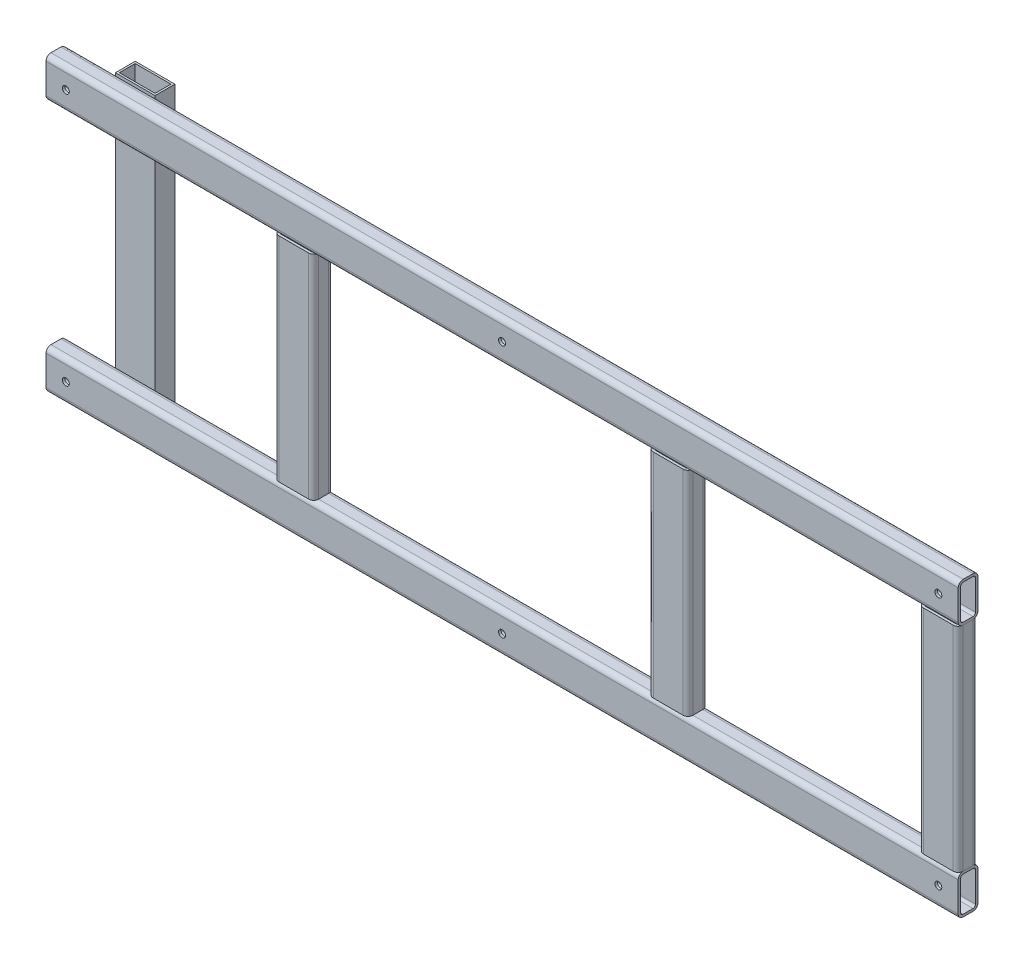
from build123d import *

# Parameters (mm, degrees)
RECT_TUBE_40X20X2_5_1_DEPTH   = 920
RECT_TUBE_40X20X2_5_1_2_DEPTH = 920
RECT_TUBE_40X20X2_5_1_3_DEPTH = 257
RECT_TUBE_40X20X2_5_1_4_DEPTH = 257
RECT_TUBE_40X20X2_5_1_5_DEPTH = 257
M6_CLEARANCE_HOLE1_AT_2_COUNT = 2
M6_CLEARANCE_HOLE1_AT_2_PITCH = 255
M6_CLEARANCE_HOLE1_AT_3_COUNT = 2
M6_CLEARANCE_HOLE1_AT_3_PITCH = 508.551865595
M6_CLEARANCE_HOLE1_AT_4_COUNT = 2
M6_CLEARANCE_HOLE1_AT_4_PITCH = 440
M6_CLEARANCE_HOLE1_AT_5_COUNT = 2
M6_CLEARANCE_HOLE1_AT_5_PITCH = 916.201397074
M6_CLEARANCE_HOLE1_AT_6_COUNT = 2
M6_CLEARANCE_HOLE1_AT_6_PITCH = 880
SKETCH7_W                     = 40
SKETCH7_H                     = 295
BOSS_EXTRUDE1_DEPTH           = 20
SKETCH8_W                     = 36
SKETCH8_H                     = 16
CUT_EXTRUDE1_DEPTH            = 967.604883083


with BuildPart() as part:
    # Sketch1 → Rect Tube 40X20X2.5(1) (new body)
    with BuildSketch(Plane(origin=(0, 0, 0), x_dir=(0, 0, 1), z_dir=(1, 0, 0))):
        with BuildLine():
            Line((-5, -20), (5, -20))
            ThreePointArc((5, -20), (8.535533906, -18.535533906), (10, -15))
            Line((10, -15), (10, 15))
            ThreePointArc((10, 15), (8.535533906, 18.535533906), (5, 20))
            Line((5, 20), (-5, 20))
            ThreePointArc((-5, 20), (-8.535533906, 18.535533906), (-10, 15))
            Line((-10, 15), (-10, -15))
            ThreePointArc((-10, -15), (-8.535533906, -18.535533906), (-5, -20))
        make_face()
        with BuildLine():
            Line((-5, -17.5), (5, -17.5))
            ThreePointArc((5, -17.5), (6.767766953, -16.767766953), (7.5, -15))
            Line((7.5, -15), (7.5, 15))
            ThreePointArc((7.5, 15), (6.767766953, 16.767766953), (5, 17.5))
            Line((5, 17.5), (-5, 17.5))
            ThreePointArc((-5, 17.5), (-6.767766953, 16.767766953), (-7.5, 15))
            Line((-7.5, 15), (-7.5, -15))
            ThreePointArc((-7.5, -15), (-6.767766953, -16.767766953), (-5, -17.5))
        make_face(mode=Mode.SUBTRACT)
    extrude(amount=RECT_TUBE_40X20X2_5_1_DEPTH)


with BuildPart() as body_2:
    # Sketch1 on segment 2 (carried to segment 2) → Rect Tube 40X20X2.5_1 2 (new body)
    with BuildSketch(Plane(origin=(0, -255, 0), x_dir=(0, 0, 1), z_dir=(1, 0, 0))):
        with BuildLine():
            Line((-5, -20), (5, -20))
            ThreePointArc((5, -20), (8.535533906, -18.535533906), (10, -15))
            Line((10, -15), (10, 15))
            ThreePointArc((10, 15), (8.535533906, 18.535533906), (5, 20))
            Line((5, 20), (-5, 20))
            ThreePointArc((-5, 20), (-8.535533906, 18.535533906), (-10, 15))
            Line((-10, 15), (-10, -15))
            ThreePointArc((-10, -15), (-8.535533906, -18.535533906), (-5, -20))
        make_face()
        with BuildLine():
            Line((-5, -17.5), (5, -17.5))
            ThreePointArc((5, -17.5), (6.767766953, -16.767766953), (7.5, -15))
            Line((7.5, -15), (7.5, 15))
            ThreePointArc((7.5, 15), (6.767766953, 16.767766953), (5, 17.5))
            Line((5, 17.5), (-5, 17.5))
            ThreePointArc((-5, 17.5), (-6.767766953, 16.767766953), (-7.5, 15))
            Line((-7.5, 15), (-7.5, -15))
            ThreePointArc((-7.5, -15), (-6.767766953, -16.767766953), (-5, -17.5))
        make_face(mode=Mode.SUBTRACT)
    extrude(amount=RECT_TUBE_40X20X2_5_1_2_DEPTH)

    # Sketch4 → M6 Clearance Hole1 (revolve, cut)
    with BuildSketch(Plane(origin=(20, -255, 10), x_dir=(0, -1, 0), z_dir=(1, 0, 0))):
        Polygon((0, 0), (0, 21.853012167), (3.5, 19.75), (3.5, 0), align=None)
    m6_clearance_hole1 = revolve(axis=Axis((20, -255, 16.35), (0, 0, -1)), mode=Mode.SUBTRACT)

    # M6 Clearance Hole1 at 4: M6 Clearance Hole1 ×2
    with Locations(*[(i * M6_CLEARANCE_HOLE1_AT_4_PITCH, 0, 0) for i in range(1, M6_CLEARANCE_HOLE1_AT_4_COUNT)]):
        add(m6_clearance_hole1, mode=Mode.SUBTRACT)

    # M6 Clearance Hole1 at 6: M6 Clearance Hole1 ×2
    with Locations(*[(i * M6_CLEARANCE_HOLE1_AT_6_PITCH, 0, 0) for i in range(1, M6_CLEARANCE_HOLE1_AT_6_COUNT)]):
        add(m6_clearance_hole1, mode=Mode.SUBTRACT)


with BuildPart() as body_3:
    # Sketch1 on segment 3 (carried to segment 3) → Rect Tube 40X20X2.5_1 3 (new body)
    with BuildSketch(Plane(origin=(900, 1, 0), x_dir=(0, 0, 1), z_dir=(0, -1, 0))):
        with BuildLine():
            Line((-5, -20), (5, -20))
            ThreePointArc((5, -20), (8.535533906, -18.535533906), (10, -15))
            Line((10, -15), (10, 15))
            ThreePointArc((10, 15), (8.535533906, 18.535533906), (5, 20))
            Line((5, 20), (-5, 20))
            ThreePointArc((-5, 20), (-8.535533906, 18.535533906), (-10, 15))
            Line((-10, 15), (-10, -15))
            ThreePointArc((-10, -15), (-8.535533906, -18.535533906), (-5, -20))
        make_face()
        with BuildLine():
            Line((-5, -17.5), (5, -17.5))
            ThreePointArc((5, -17.5), (6.767766953, -16.767766953), (7.5, -15))
            Line((7.5, -15), (7.5, 15))
            ThreePointArc((7.5, 15), (6.767766953, 16.767766953), (5, 17.5))
            Line((5, 17.5), (-5, 17.5))
            ThreePointArc((-5, 17.5), (-6.767766953, 16.767766953), (-7.5, 15))
            Line((-7.5, 15), (-7.5, -15))
            ThreePointArc((-7.5, -15), (-6.767766953, -16.767766953), (-5, -17.5))
        make_face(mode=Mode.SUBTRACT)
    extrude(amount=RECT_TUBE_40X20X2_5_1_3_DEPTH)

    # Rect Tube 40X20X2.5_1 3 end butt 1
    split(bisect_by=Plane(origin=(900, -20, 0), x_dir=(1, 0, 0), z_dir=(0, -1, 0)), keep=Keep.TOP)

    # Rect Tube 40X20X2.5_1 3 end butt 2
    split(bisect_by=Plane(origin=(900, -235, 0), x_dir=(-1, 0, 0), z_dir=(0, 1, 0)), keep=Keep.TOP)


with BuildPart() as body_4:
    # Sketch1 on segment 4 (carried to segment 4) → Rect Tube 40X20X2.5_1 4 (new body)
    with BuildSketch(Plane(origin=(250, 1, 0), x_dir=(0, 0, 1), z_dir=(0, -1, 0))):
        with BuildLine():
            Line((-5, -20), (5, -20))
            ThreePointArc((5, -20), (8.535533906, -18.535533906), (10, -15))
            Line((10, -15), (10, 15))
            ThreePointArc((10, 15), (8.535533906, 18.535533906), (5, 20))
            Line((5, 20), (-5, 20))
            ThreePointArc((-5, 20), (-8.535533906, 18.535533906), (-10, 15))
            Line((-10, 15), (-10, -15))
            ThreePointArc((-10, -15), (-8.535533906, -18.535533906), (-5, -20))
        make_face()
        with BuildLine():
            Line((-5, -17.5), (5, -17.5))
            ThreePointArc((5, -17.5), (6.767766953, -16.767766953), (7.5, -15))
            Line((7.5, -15), (7.5, 15))
            ThreePointArc((7.5, 15), (6.767766953, 16.767766953), (5, 17.5))
            Line((5, 17.5), (-5, 17.5))
            ThreePointArc((-5, 17.5), (-6.767766953, 16.767766953), (-7.5, 15))
            Line((-7.5, 15), (-7.5, -15))
            ThreePointArc((-7.5, -15), (-6.767766953, -16.767766953), (-5, -17.5))
        make_face(mode=Mode.SUBTRACT)
    extrude(amount=RECT_TUBE_40X20X2_5_1_4_DEPTH)

    # Rect Tube 40X20X2.5_1 4 end butt 1
    split(bisect_by=Plane(origin=(250, -20, 0), x_dir=(1, 0, 0), z_dir=(0, -1, 0)), keep=Keep.TOP)

    # Rect Tube 40X20X2.5_1 4 end butt 2
    split(bisect_by=Plane(origin=(250, -235, 0), x_dir=(-1, 0, 0), z_dir=(0, 1, 0)), keep=Keep.TOP)


with BuildPart() as body_5:
    # Sketch1 on segment 5 (carried to segment 5) → Rect Tube 40X20X2.5_1 5 (new body)
    with BuildSketch(Plane(origin=(627.472616431, 1, 0), x_dir=(0, 0, 1), z_dir=(0, -1, 0))):
        with BuildLine():
            Line((-5, -20), (5, -20))
            ThreePointArc((5, -20), (8.535533906, -18.535533906), (10, -15))
            Line((10, -15), (10, 15))
            ThreePointArc((10, 15), (8.535533906, 18.535533906), (5, 20))
            Line((5, 20), (-5, 20))
            ThreePointArc((-5, 20), (-8.535533906, 18.535533906), (-10, 15))
            Line((-10, 15), (-10, -15))
            ThreePointArc((-10, -15), (-8.535533906, -18.535533906), (-5, -20))
        make_face()
        with BuildLine():
            Line((-5, -17.5), (5, -17.5))
            ThreePointArc((5, -17.5), (6.767766953, -16.767766953), (7.5, -15))
            Line((7.5, -15), (7.5, 15))
            ThreePointArc((7.5, 15), (6.767766953, 16.767766953), (5, 17.5))
            Line((5, 17.5), (-5, 17.5))
            ThreePointArc((-5, 17.5), (-6.767766953, 16.767766953), (-7.5, 15))
            Line((-7.5, 15), (-7.5, -15))
            ThreePointArc((-7.5, -15), (-6.767766953, -16.767766953), (-5, -17.5))
        make_face(mode=Mode.SUBTRACT)
    extrude(amount=RECT_TUBE_40X20X2_5_1_5_DEPTH)

    # Rect Tube 40X20X2.5_1 5 end butt 1
    split(bisect_by=Plane(origin=(627.472616431, -20, 0), x_dir=(1, 0, 0), z_dir=(0, -1, 0)), keep=Keep.TOP)

    # Rect Tube 40X20X2.5_1 5 end butt 2
    split(bisect_by=Plane(origin=(627.472616431, -235, 0), x_dir=(-1, 0, 0), z_dir=(0, 1, 0)), keep=Keep.TOP)


with BuildPart() as part_1:
    add(part.part)

    # M6 Clearance Hole1 at 2: M6 Clearance Hole1 ×2
    with Locations(*[(0, i * M6_CLEARANCE_HOLE1_AT_2_PITCH, 0) for i in range(1, M6_CLEARANCE_HOLE1_AT_2_COUNT)]):
        add(m6_clearance_hole1, mode=Mode.SUBTRACT)

    # M6 Clearance Hole1 at 3: M6 Clearance Hole1 ×2
    with Locations(*[Vector(0.8652018206350236, 0.5014237824134796, 0) * (i * M6_CLEARANCE_HOLE1_AT_3_PITCH) for i in range(1, M6_CLEARANCE_HOLE1_AT_3_COUNT)]):
        add(m6_clearance_hole1, mode=Mode.SUBTRACT)

    # M6 Clearance Hole1 at 5: M6 Clearance Hole1 ×2
    with Locations(*[Vector(0.9604875116001456, 0.2783230857477695, 0) * (i * M6_CLEARANCE_HOLE1_AT_5_PITCH) for i in range(1, M6_CLEARANCE_HOLE1_AT_5_COUNT)]):
        add(m6_clearance_hole1, mode=Mode.SUBTRACT)


with BuildPart() as body_6:
    # Sketch7 → Boss-Extrude1 (new body)
    with BuildSketch(Plane.XY.offset(-10)):
        with Locations((70, -127.5)):
            Rectangle(SKETCH7_W, SKETCH7_H)
    extrude(amount=-BOSS_EXTRUDE1_DEPTH)

    # Sketch8 → Cut-Extrude1 (cut, through all)
    with BuildSketch(Plane(origin=(0, 20, 0), x_dir=(1, 0, 0), z_dir=(0, 1, 0))):
        with Locations((70, 20)):
            Rectangle(SKETCH8_W, SKETCH8_H)
    extrude(amount=-CUT_EXTRUDE1_DEPTH, mode=Mode.SUBTRACT)


solid = Compound([body_2.part, body_3.part, body_4.part, body_5.part, part_1.part, body_6.part])
